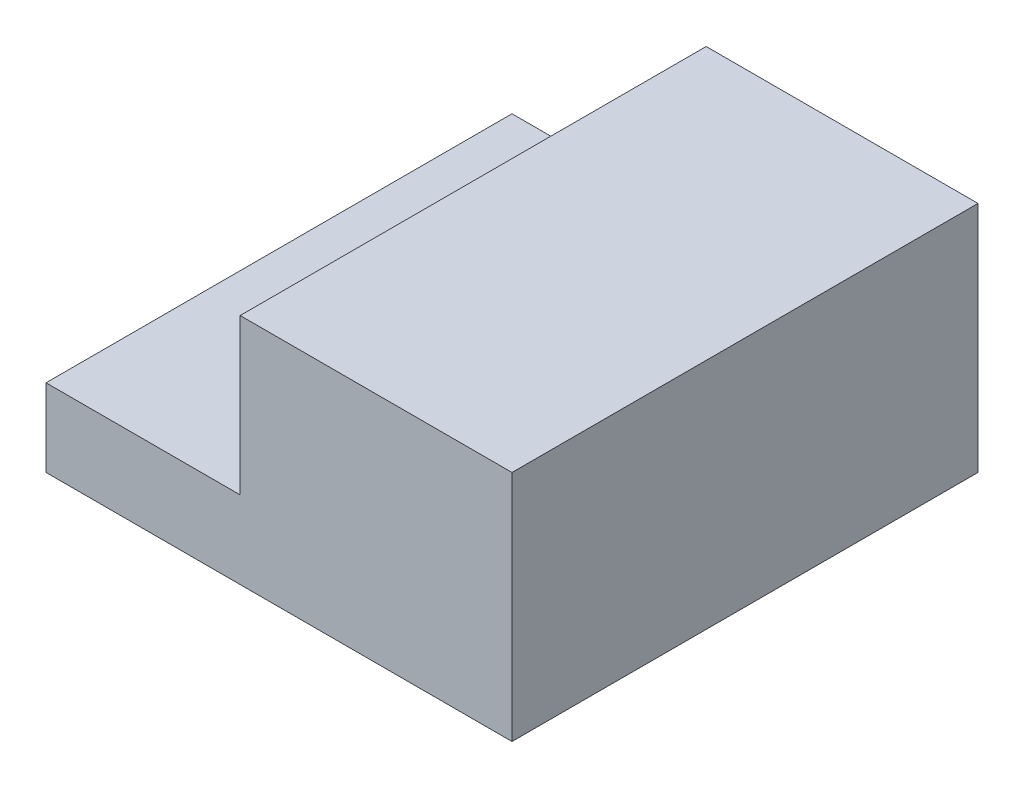
from build123d import *

# Parameters (mm, degrees)
EXTRUDE_1_DEPTH = 300


with BuildPart() as part:
    # 草图1 → 凸台-拉伸1 (new, symmetric)
    with BuildSketch(Plane.XY):
        Polygon((0, 0), (0, 100), (250, 100), (250, 300), (600, 300), (600, 0), align=None)
    extrude(amount=EXTRUDE_1_DEPTH, both=True)


solid = part.part
